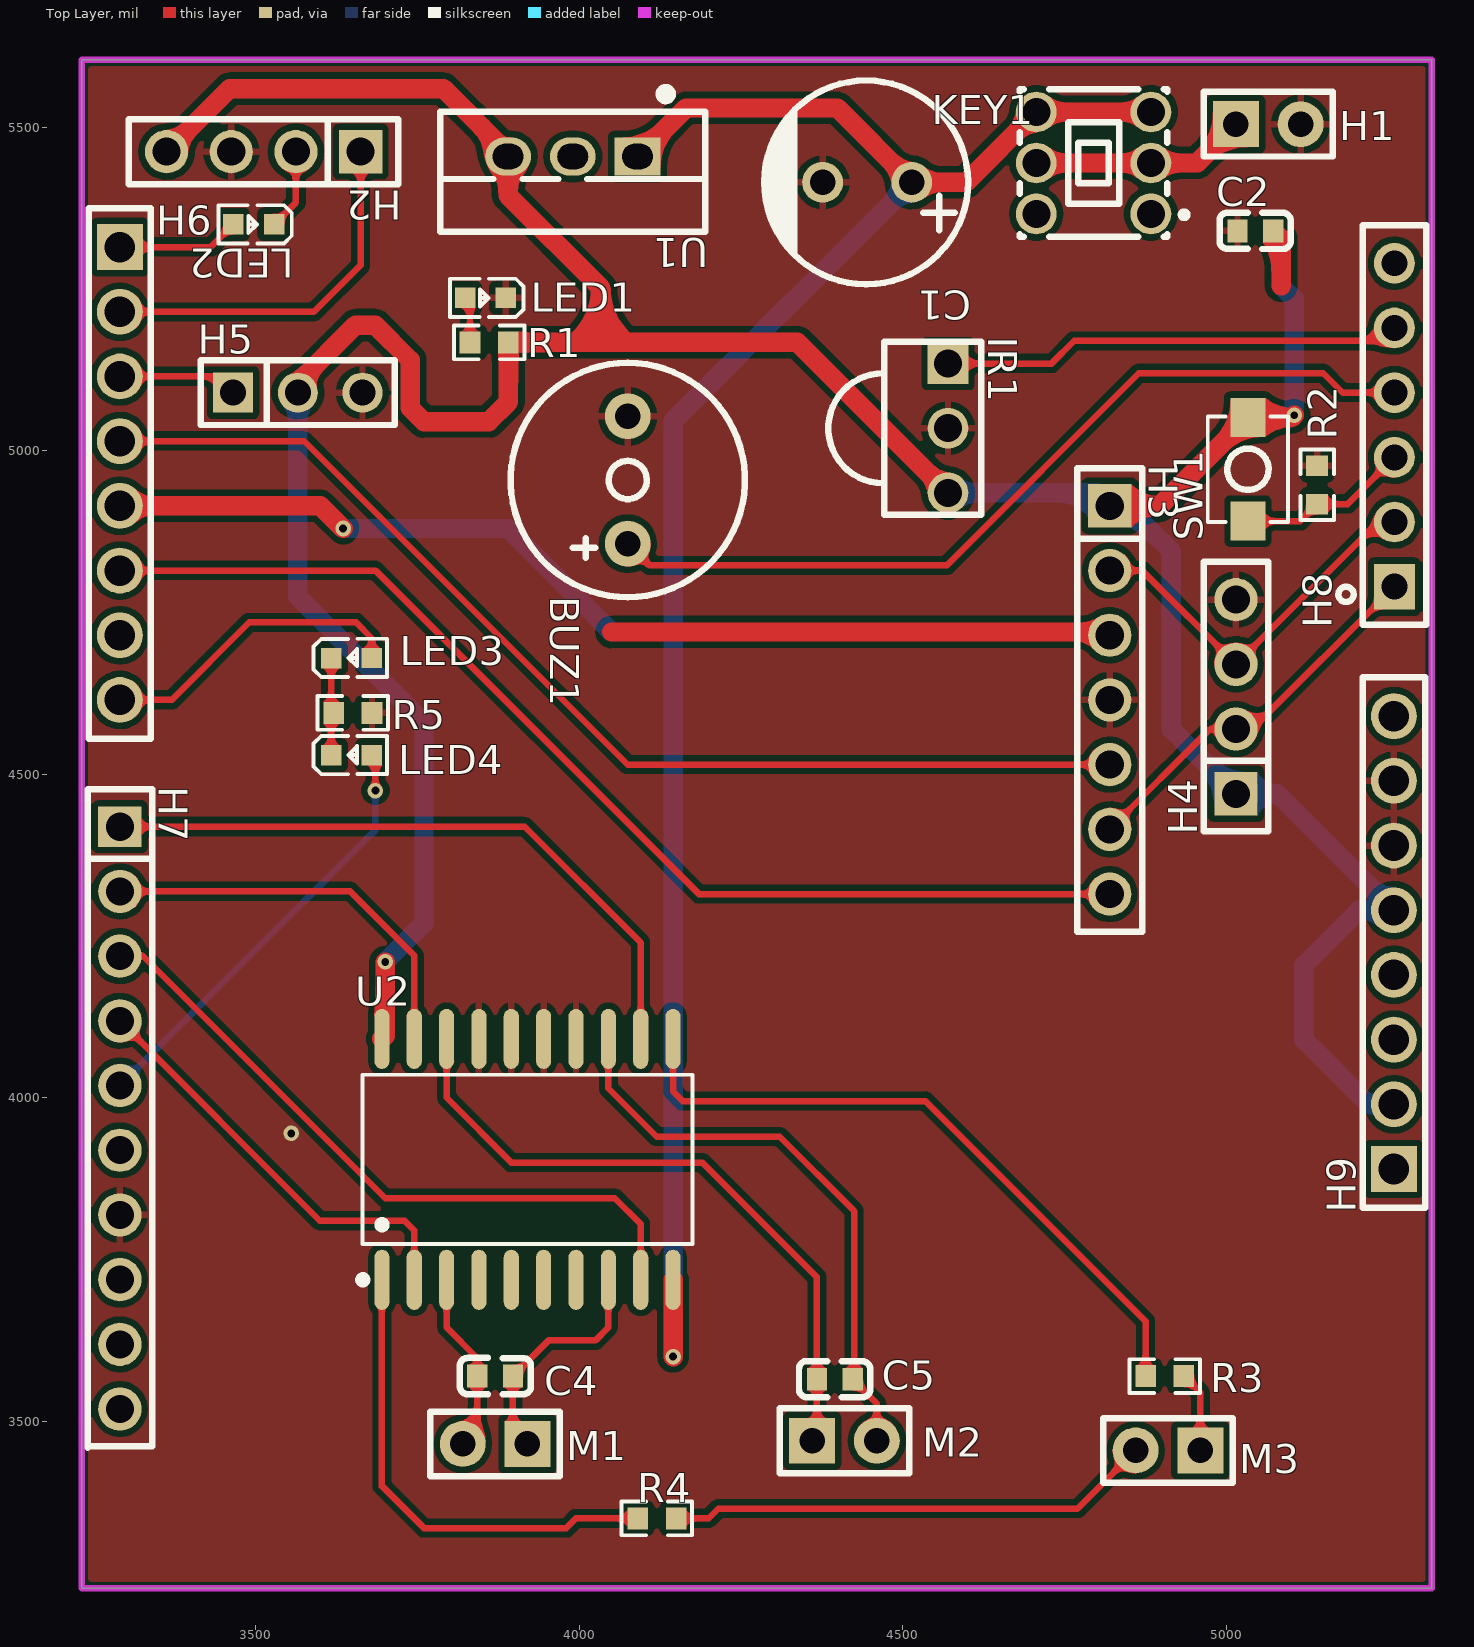
[diagram p0: Top Layer view]
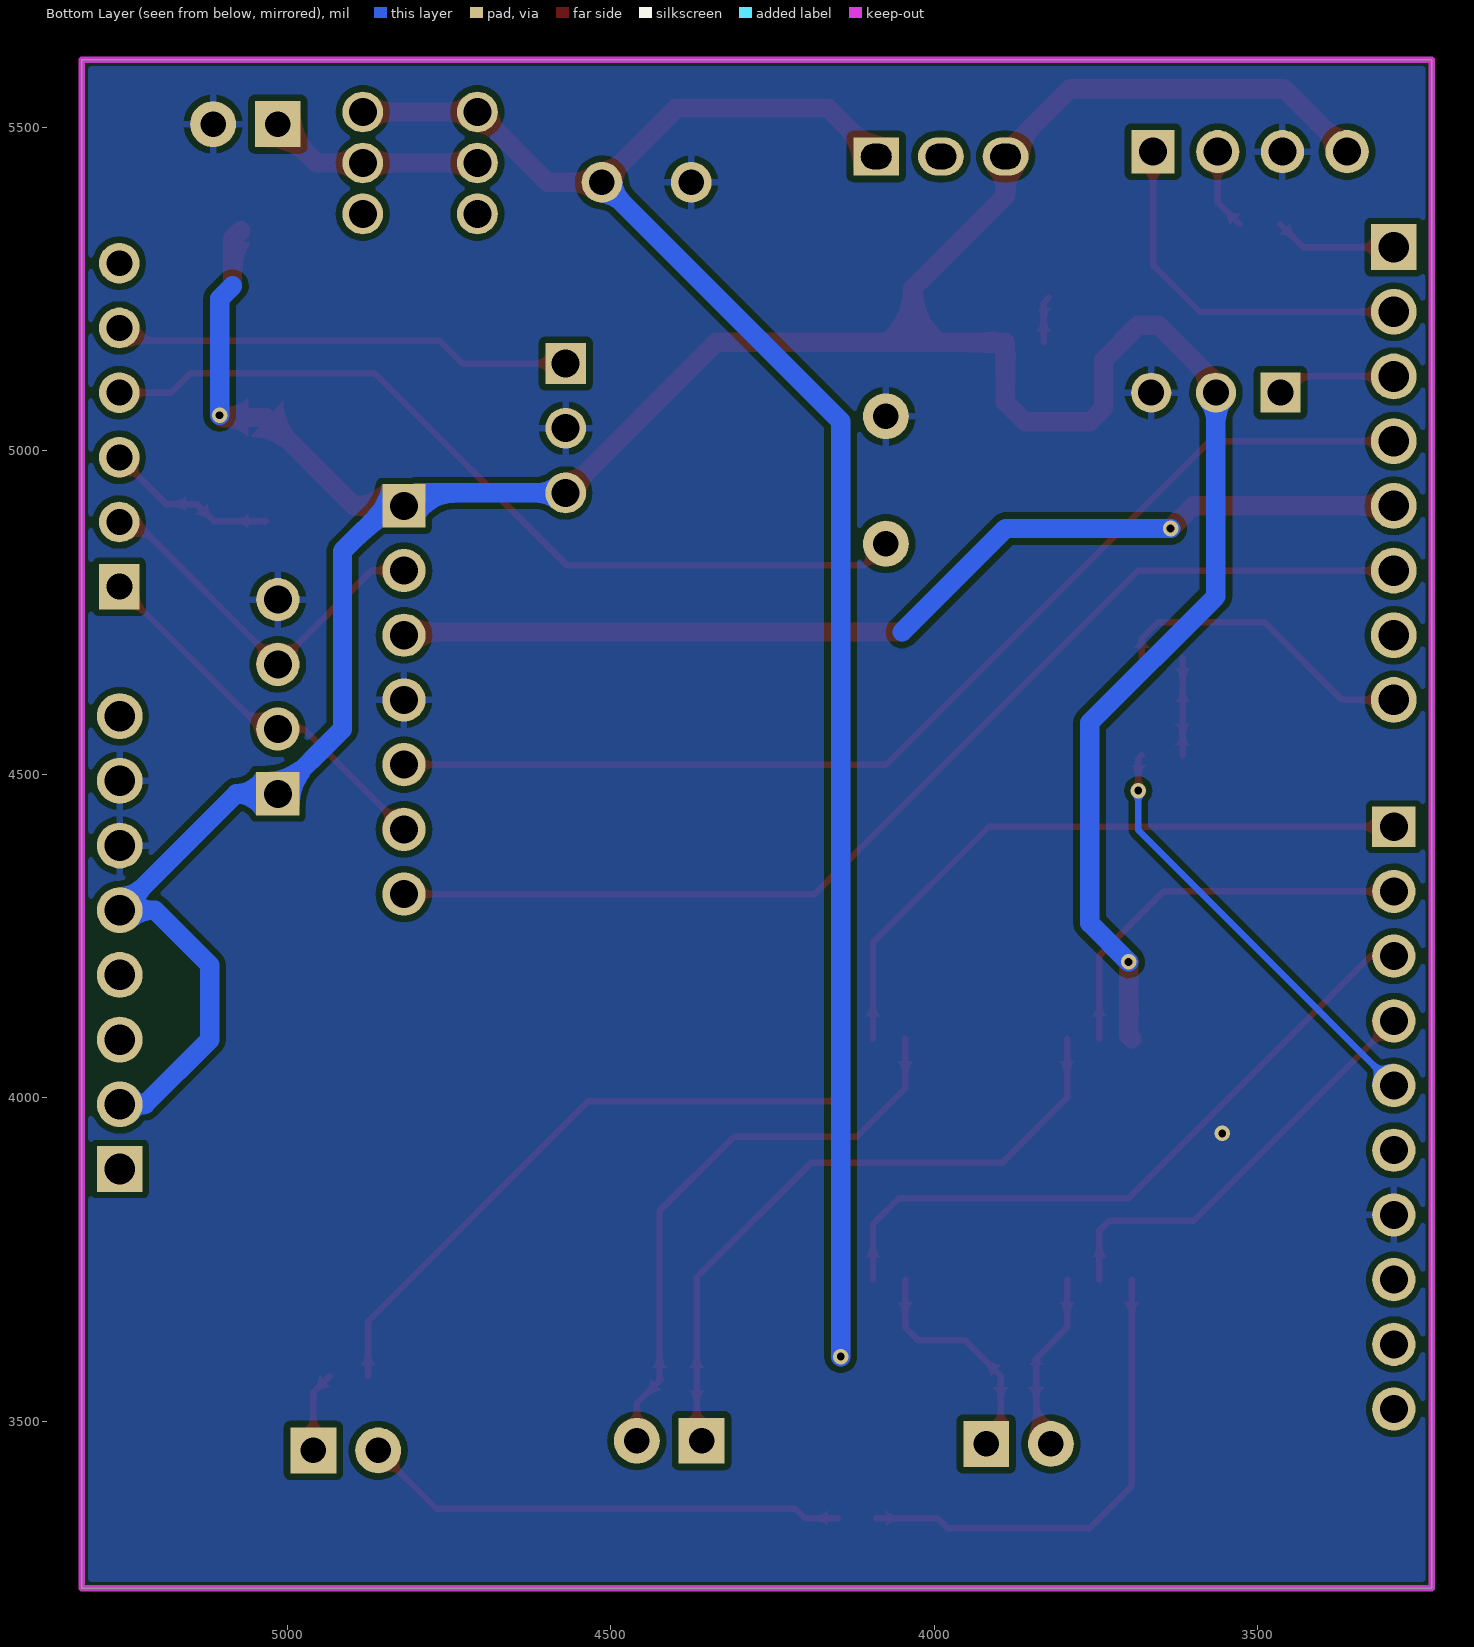
[diagram p1: Bottom Layer view, seen from below]
# Altium PCB MISC51932.pcbdoc
Units mil, origin at the board's own origin, x right, y up, seen from the top; angles counter-clockwise.
Board outline 2086.61 x 2362.2 mil, 2 copper layers (Top Layer, Bottom Layer), stack 62.206 mil thick; 31 components, 32 nets, 120 pads, 6 vias.

## Layer stack, top to bottom
Top Solder Mask Layer: solder mask 0.394, Dk 3.3
Top Layer: signal copper 1.379
Dielectric1: surface 59.449, FR4, Dk 4.5
Bottom Layer: signal copper 1.378
Bottom Solder Mask Layer: solder mask 0.394, Dk 3.3

## Board outline
5317.83,5604.37 3231.22,5604.37 3231.22,3242.17 5317.83,3242.17

## Design rules (kind name [scope] priority, off if disabled: settings)
BoardOutlineClearance copperThickness2oz_1 [All] p2 off: genericclearance=7.99 ignorepadtopadclearanceinfootprint=FALSE except(0: Arc-SplitContinuation Track-SplitContinuation SMDPad-SplitContinuation THPad-SplitContinuation Via-SplitContinuation Fill-SplitContinuation Region-SplitContinuation Poly-SplitContinuation Text-SplitContinuation Hole-SplitContinuation; 5.98: Arc-CutoutEdge Track-CutoutEdge SMDPad-CutoutEdge THPad-CutoutEdge Via-CutoutEdge Text-CutoutEdge; 6.9: Hole-OutlineEdge Hole-CutoutEdge; 10: Poly-OutlineEdge Poly-CutoutEdge; 11.81: Arc-OutlineEdge Track-OutlineEdge SMDPad-OutlineEdge THPad-OutlineEdge Via-OutlineEdge Fill-OutlineEdge Region-OutlineEdge Text-OutlineEdge Fill-CutoutEdge Region-CutoutEdge)
BoardOutlineClearance Plane_innerPlane_1 [All] p4 off: genericclearance=4.02 ignorepadtopadclearanceinfootprint=FALSE except(0: Arc-SplitContinuation Track-SplitContinuation SMDPad-SplitContinuation THPad-SplitContinuation Via-SplitContinuation Fill-SplitContinuation Region-SplitContinuation Poly-SplitContinuation Text-SplitContinuation Hole-SplitContinuation; 5.98: Arc-CutoutEdge Track-CutoutEdge SMDPad-CutoutEdge THPad-CutoutEdge Via-CutoutEdge Text-CutoutEdge; 6.9: Hole-OutlineEdge Hole-CutoutEdge; 10: Poly-OutlineEdge Poly-CutoutEdge; 11.81: Arc-OutlineEdge Track-OutlineEdge SMDPad-OutlineEdge THPad-OutlineEdge Via-OutlineEdge Fill-OutlineEdge Region-OutlineEdge Text-OutlineEdge Fill-CutoutEdge Region-CutoutEdge)
BoardOutlineClearance Copper_copperRegion_1 [All] p6 off: genericclearance=4.02 ignorepadtopadclearanceinfootprint=FALSE except(0: Arc-SplitContinuation Track-SplitContinuation SMDPad-SplitContinuation THPad-SplitContinuation Via-SplitContinuation Fill-SplitContinuation Region-SplitContinuation Poly-SplitContinuation Text-SplitContinuation Hole-SplitContinuation; 5.98: Arc-CutoutEdge Track-CutoutEdge SMDPad-CutoutEdge THPad-CutoutEdge Via-CutoutEdge Text-CutoutEdge; 6.9: Hole-OutlineEdge Hole-CutoutEdge; 10: Poly-OutlineEdge Poly-CutoutEdge; 11.81: Arc-OutlineEdge Track-OutlineEdge SMDPad-OutlineEdge THPad-OutlineEdge Via-OutlineEdge Fill-OutlineEdge Region-OutlineEdge Text-OutlineEdge Fill-CutoutEdge Region-CutoutEdge)
BoardOutlineClearance copperThickness1oz_1 [All] p8: genericclearance=4.02 ignorepadtopadclearanceinfootprint=FALSE except(0: Arc-SplitContinuation Track-SplitContinuation SMDPad-SplitContinuation THPad-SplitContinuation Via-SplitContinuation Fill-SplitContinuation Region-SplitContinuation Poly-SplitContinuation Text-SplitContinuation Hole-SplitContinuation; 5.98: Arc-CutoutEdge Track-CutoutEdge SMDPad-CutoutEdge THPad-CutoutEdge Via-CutoutEdge Text-CutoutEdge; 6.9: Hole-OutlineEdge Hole-CutoutEdge; 10: Poly-OutlineEdge Poly-CutoutEdge; 11.81: Arc-OutlineEdge Track-OutlineEdge SMDPad-OutlineEdge THPad-OutlineEdge Via-OutlineEdge Fill-OutlineEdge Region-OutlineEdge Text-OutlineEdge Fill-CutoutEdge Region-CutoutEdge)
Clearance copperThickness2oz [All] p1 off: gap=7.99 ignorepadtopadclearanceinfootprint=FALSE except(5.98: SMDPad-Track SMDPad-SMDPad THPad-Track SMDPad-THPad THPad-THPad Track-Via SMDPad-Via THPad-Via Via-Via Fill-SMDPad Region-SMDPad Fill-THPad Region-THPad Fill-Via Region-Via Fill-Fill Fill-Region Region-Region Arc-Track Arc-SMDPad Arc-THPad Arc-Via Fill-Arc Region-Arc Arc-Arc Text-Track SMDPad-Text Text-THPad Text-Via Fill-Text Region-Text Arc-Text Text-Text; 6.9: Hole-Track Hole-SMDPad Hole-THPad Hole-Via Fill-Hole Region-Hole Hole-Arc Hole-Text; 10: Poly-Track Poly-SMDPad Poly-THPad Poly-Via Poly-Fill Poly-Region Poly-Poly Poly-Arc Poly-Text Poly-Hole; 11.81: Fill-Track Region-Track)
Clearance Plane_innerPlane [All] p3 off: gap=4.02 ignorepadtopadclearanceinfootprint=FALSE except(5.98: SMDPad-Track SMDPad-SMDPad THPad-Track SMDPad-THPad THPad-THPad Track-Via SMDPad-Via THPad-Via Via-Via Fill-SMDPad Region-SMDPad Fill-THPad Region-THPad Fill-Via Region-Via Fill-Fill Fill-Region Region-Region Arc-Track Arc-SMDPad Arc-THPad Arc-Via Fill-Arc Region-Arc Arc-Arc Text-Track SMDPad-Text Text-THPad Text-Via Fill-Text Region-Text Arc-Text Text-Text; 6.9: Hole-Track Hole-SMDPad Hole-THPad Hole-Via Fill-Hole Region-Hole Hole-Arc Hole-Text; 10: Poly-Track Poly-SMDPad Poly-THPad Poly-Via Poly-Fill Poly-Region Poly-Poly Poly-Arc Poly-Text Poly-Hole; 11.81: Fill-Track Region-Track)
Clearance Copper_copperRegion [All] p5 off: gap=4.02 ignorepadtopadclearanceinfootprint=FALSE except(5.98: SMDPad-Track SMDPad-SMDPad THPad-Track SMDPad-THPad THPad-THPad Track-Via SMDPad-Via THPad-Via Via-Via Fill-SMDPad Region-SMDPad Fill-THPad Region-THPad Fill-Via Region-Via Fill-Fill Fill-Region Region-Region Arc-Track Arc-SMDPad Arc-THPad Arc-Via Fill-Arc Region-Arc Arc-Arc Text-Track SMDPad-Text Text-THPad Text-Via Fill-Text Region-Text Arc-Text Text-Text; 6.9: Hole-Track Hole-SMDPad Hole-THPad Hole-Via Fill-Hole Region-Hole Hole-Arc Hole-Text; 10: Poly-Track Poly-SMDPad Poly-THPad Poly-Via Poly-Fill Poly-Region Poly-Poly Poly-Arc Poly-Text Poly-Hole; 11.81: Fill-Track Region-Track)
Clearance copperThickness1oz [All] p7: gap=4.02 ignorepadtopadclearanceinfootprint=FALSE except(5.98: SMDPad-Track SMDPad-SMDPad THPad-Track SMDPad-THPad THPad-THPad Track-Via SMDPad-Via THPad-Via Via-Via Fill-SMDPad Region-SMDPad Fill-THPad Region-THPad Fill-Via Region-Via Fill-Fill Fill-Region Region-Region Arc-Track Arc-SMDPad Arc-THPad Arc-Via Fill-Arc Region-Arc Arc-Arc Text-Track SMDPad-Text Text-THPad Text-Via Fill-Text Region-Text Arc-Text Text-Text; 6.9: Hole-Track Hole-SMDPad Hole-THPad Hole-Via Fill-Hole Region-Hole Hole-Arc Hole-Text; 10: Poly-Track Poly-SMDPad Poly-THPad Poly-Via Poly-Fill Poly-Region Poly-Poly Poly-Arc Poly-Text Poly-Hole; 11.81: Fill-Track Region-Track)
DiffPairsRouting differentialPair [All] p1: maxlimit=6 minlimit=6 mostfreqgap=6 toplayer_minwidth=5 toplayer_prefwidth=10 toplayer_maxwidth=100 toplayer_mingap=6 toplayer_prefgap=6 toplayer_maxgap=6 bottomlayer_minwidth=5 bottomlayer_prefwidth=10 bottomlayer_maxwidth=100 bottomlayer_mingap=6 bottomlayer_prefgap=6 bottomlayer_maxgap=6 maxuncoupledlength=10
HoleToHoleClearance otherClearance [All] p1: gap=11.81 allowstackedmicrovias=TRUE
Length netLength [All] p1: minlimit=0 maxlimit=0
PasteMaskExpansion pasteMaskExpansion [All] p1: expansion=0
PlaneConnect innerPlane [All] p1: planeconnectstyle=Relief reliefexpansion=20 reliefentries=4 reliefconductorwidth=10 reliefairgap=10
PolygonConnect copperRegion [All] p1: connectstyle=Relief reliefconductorwidth=10 reliefentries=4 polygonreliefangle="90 Angle" airgapwidth=10 via.connectstyle=Relief via.reliefconductorwidth=10 via.reliefentries=4 via.polygonreliefangle="90 Angle" via.airgapwidth=10
RoutingVias viaSize [All] p1: holewidth=12.01 width=24.02 viastyle="Through Hole" minholewidth=11.81 minwidth=19.68 maxholewidth=248.03 maxwidth=393.7
SolderMaskExpansion solderMaskExpansion [IsVia] p1: expansion=-1000 istentingtop=TRUE
SolderMaskExpansion solderMaskExpansion [All] p2: expansion=2 istentingtop=FALSE
Width copperThickness2oz_2 [All] p1 off: maxlimit=100 minlimit=8 preferedwidth=10
Width copperThickness1oz_2 [All] p2: maxlimit=100 minlimit=5 preferedwidth=10

## Components (designator, comment, footprint, x,y, rotation, side; value= is the part's Value field where it differs from the comment)
BUZ1 "蜂鸣器" BUZ-TH_BD9.0-P5.00-D0.6-FD 4075,4955 r90 top
C1 "1000uF" CAP-TH_BD8.0-P3.50-D0.6-FD 4445,5415 r180 top
C2 "100nF" C0603 5045,5340 r0 top
C4 "100nF" C0603 3870,3570 r180 top
C5 "100nF" C0603 4395,3565 r0 top
H1 "" HDR-TH_2P-P2.54-V-M-1 5065,5505 r0 top
H2 "" HDR-TH_4P-P2.54-V-F 3512.13,5462.4 r180 top
H3 "" HDR-TH_7P-P2.54-V-M 4820,4615 r270 top
H4 "" HDR-TH_4P-P2.54-V-F 5015,4620 r90 top
H5 "" HDR-TH_3P-P2.54-V-F 3565,5090 r0 top
H6 "" HDR-TH_8P-P2.54-V-F-1 3290,4965 r270 top
H7 "" HDR-TH_10P-P2.54-V-F 3290,3969.02 r270 top
H8 "" HDR-TH_6P-P2.54-V-F 5260,5040 r90 top
H9 "" HDR-TH_8P-P2.54-V-F-1 5259.27,4240 r90 top
IR1 "IRM-8601M2(GPS)" SENSOR-TH_IRM-8601 4570,5035 r270 top
KEY1 "自锁开关 5.8Z白灰白260G" SW-TH_6P-L5.8-W5.8-P2.00-LS4.5-TR 4795,5445 r270 top
LED1 "" LED_0603 3853.12,5236.36 r180 top
LED2 "" LED_0603 3495,5350 r180 top
LED3 "" LED_0603 3650,4680 r0 top
LED4 "" LED_0603 3650,4530 r0 top
M1 "" HDR-TH_2P-P2.54-V-M-1 3870,3465 r180 top
M2 "" HDR-TH_2P-P2.54-V-M-1 4410,3470 r0 top
M3 "" HDR-TH_2P-P2.54-V-M-1 4910,3455 r180 top
R1 "4.7K" R0603 3860.83,5167.59 r0 top
R2 "4.7K" R0603 5140.59,4947.46 r270 top
R3 "1K" R0603 4905,3570 r0 top
R4 "1K" R0603 4120,3350 r0 top
R5 "4.7K" R0603 3650,4595 r0 top
SW1 "" Key_SMD_3x4x2 5033.58,4971.53 r90 top
U1 "7805" TO-220-3_L10.2-W4.5-P2.54-L-1 3990,5455 r180 top
U2 "L293DD" SOIC-20_L13.0-W7.6-P1.27-LS10.3-BL 3920,3905 r0 top

## Footprints (in the part's own frame and the unit in brackets; to place one, negate y for a bottom-side part, rotate by r counter-clockwise, add the part's x,y. Pads: shape width x height; smd on the part's side, far side on the other; paste and mask are expansions set on the pad)
BUZ-TH_BD9.0-P5.00-D0.6-FD [mm]
  round 1.8 hole 1 copper offset 0,0: 1(-2.5,0)
  round 1.8 hole 1: 2(2.5,0)
  silkscreen extent -4.6,-4.6 4.6,4.6
C0603 [mm]
  rect 0.8x0.9 smd: 1(-0.7,0) 2(0.7,0)
  silkscreen extent -1.41,-0.71 1.39,0.72
CAP-TH_BD8.0-P3.50-D0.6-FD [mm]
  round 1.6 hole 1: 1(-1.75,0) 2(1.75,0)
  silkscreen extent -3.96,-4 4.04,4
HDR-TH_2P-P2.54-V-M-1 [mm]
  rect 1.8x1.8 hole 1: 1(-1.27,0)
  round 1.8 hole 1: 2(1.27,0)
  silkscreen extent -2.54,-1.27 2.54,1.27
HDR-TH_3P-P2.54-V-F [mil]
  rect 62x62 hole 40.16: 1(-100,0)
  round 62 hole 40.16: 2(0,0) 3(100,0)
  silkscreen extent -150,-50 150,50
HDR-TH_4P-P2.54-V-F [mm]
  rect 1.7x1.7 hole 1.1: 1(-3.81,0)
  round 1.7 hole 1.1: 2(-1.27,0) 3(1.27,0) 4(3.81,0)
  silkscreen extent -5.29,-1.27 5.29,1.27
HDR-TH_6P-P2.54-V-F [mm]
  rect 1.8x1.6 hole 1.02: 1(-6.35,0)
  round 1.6 hole 1.02: 2(-3.81,0) 3(-1.27,0) 4(1.27,0) 5(3.81,0) 6(6.35,0)
  silkscreen extent -7.85,-1.25 7.85,2.2
HDR-TH_7P-P2.54-V-M [mm]
  rect 1.7x1.7 hole 1.1: 1(-7.62,0)
  round 1.7 hole 1.1: 2(-5.08,0) 3(-2.54,0) 4(0,0) 5(2.54,0) 6(5.08,0) 7(7.62,0)
  silkscreen extent -9.1,-1.27 9.1,1.27
HDR-TH_8P-P2.54-V-F-1 [mm]
  rect 1.8x1.8 hole 1.2: 1(-8.89,0)
  round 1.8 hole 1.2: 2(-6.35,0) 3(-3.81,0) 4(-1.27,0) 5(1.27,0) 6(3.81,0) 7(6.35,0) 8(8.89,0)
  silkscreen extent -10.41,-1.22 10.41,1.22
HDR-TH_10P-P2.54-V-F [mm]
  rect 1.575x1.7 hole 1.1: 1(-11.43,0)
  round 1.7 hole 1.1: 2(-8.89,0) 3(-6.35,0) 4(-3.81,0) 5(-1.27,0) 6(1.27,0) 7(3.81,0) 8(6.35,0) 9(8.89,0) 10(11.43,0)
  silkscreen extent -12.9,-1.27 12.95,1.27
Key_SMD_3x4x2 [mm]
  rect 1.53x1.36 smd paste+0 mask+0.051: 1(-2.035,0) 2(2.035,0)
  silkscreen extent -2.08,-1.58 2.08,1.58
LED_0603 [mil]
  rect 31.5x31.5 smd paste+0 mask+2: 1(-33.5,-0.4) 2(29.5,-0.2)
  silkscreen extent -61,-30 53,30
R0603 [mil]
  rect 31.75x34.02 smd paste-3937.01 mask+2: 1(-29.66,0) 2(29.66,0)
  silkscreen extent -55,-26 55,26
SENSOR-TH_IRM-8601 [mm]
  rect 1.6x1.6 hole 1.1: 1(-2.54,0)
  round 1.6 hole 1.1: 2(0,0) 3(2.54,0)
  silkscreen extent -3.4,-4.7 3.4,1.3
SOIC-20_L13.0-W7.6-P1.27-LS10.3-BL [mm]
  oval 0.595x2.36 smd: 1(-5.715,-4.73) 2(-4.445,-4.73) 3(-3.175,-4.73) 4(-1.905,-4.73) 5(-0.635,-4.73) 6(0.635,-4.73) 7(1.905,-4.73) 8(3.175,-4.73) 9(4.445,-4.73) 10(5.715,-4.73) 11(5.715,4.73) 12(4.445,4.73) 13(3.175,4.73) 14(1.905,4.73) 15(0.635,4.73) 16(-0.635,4.73) 17(-1.905,4.73) 18(-3.175,4.73) 19(-4.445,4.73) 20(-5.715,4.73)
  silkscreen extent -6.61,-4.88 6.48,3.32
SW-TH_6P-L5.8-W5.8-P2.00-LS4.5-TR [mm]
  round 1.6 hole 1.1: 1(2,2.25) 2(0,2.25) 3(-2,2.25) 4(-2,-2.25) 5(0,-2.25) 6(2,-2.25)
  silkscreen extent -2.9,-2.9 2.9,3.68
TO-220-3_L10.2-W4.5-P2.54-L-1 [mm]
  rect 1.8x1.5 hole 1 slot 1.2 at 0 deg: 1(-2.54,0)
  oval 1.8x1.5 hole 1 slot 1.2 at 0 deg: 2(0,0) 3(2.54,0)
  silkscreen extent -5.2,-2.65 5.2,2.95

## Via types
v1: diameter 24, hole 12, Top Layer to Bottom Layer, 5 vias
v2: diameter 24.02, hole 12, Top Layer to Bottom Layer, 1 vias

## Nets (pads, with @x,y where several pads share a name; then routed paths per layer and width w, separated by ;. In a path a pad name is that pad's centre, name@x,y a point inside that pad or via, vN(x,y) a via of type N, cw(c..) or ccw(c..) an arc to the next point about the centre after c; other vN are vias at no path point)
$1N326: LED1.2 R1.1 | length 72.1
  Top Layer w10: LED1.2 3831.17,5229.01 R1.1
$1N838: H1.1 KEY1.2 KEY1.5 | length 333.4
  Top Layer w30: KEY1.5 KEY1.2 4955,5445 H1.1
$1N1064: H2.2 LED2.1 | length 125.9
  Top Layer w10: LED2.1 3562.13,5384.03 H2.2
$1N2239: C4.1 M1.1 U2.8 | length 366.6
  Top Layer w10: M1.1 3897.56,3487.44 C4.1 3952.56,3625 4025,3625 4045,3645 U2.8
$1N2244: C4.2 M1.2 U2.3 | length 282.7
  Top Layer w10: U2.3 3795,3645 3842.44,3597.56 C4.2 3842.44,3487.44 M1.2
$1N2373: C5.1 M2.1 U2.18 | length 1034.2
  Top Layer w10: U2.18 3795,4000 3895,3900 4190,3900 4367.44,3722.56 C5.1 4367.44,3477.44 M2.1
$1N2377: C5.2 M2.2 U2.13 | length 906.4
  Top Layer w10: U2.13 4045,4015 4120,3940 4310,3940 4425,3825 4425,3567.44 C5.2 4460,3527.56 M2.2
$1N2532: R4.1 U2.1 | length 747.3
  Top Layer w10: U2.1 3695,3400 3760,3335 3980,3335 3995,3350 R4.1
$1N2537: R3.1 U2.11 | length 1043.4
  Top Layer w10: U2.11 4145,4010 4160,3995 4535,3995 4875.34,3654.66 R3.1
$1N2566: M3.1 R3.2 | length 125.5
  Top Layer w10: R3.2 4960,3544.66 M3.1
$1N2602: M3.2 R4.2 | length 753.8
  Top Layer w10: R4.2 4200,3350 4215,3365 4770,3365 M3.2
$1N3024: H6.8 LED3.2 | length 480.1
  Top Layer w10: H6.8 3370,4615 3490,4735 3655,4735 3679.5,4710.5 LED3.2
$1N3068: H7.5 LED4.2 | length 676.7
  Top Layer w10: LED4.2 3685,4524.3 v1(3685,4475)
  Bottom Layer w10: H7.5 3685,4414.02 v1(3685,4475)
$1N3103: LED3.1 LED4.1 R5.1 | length 150
  Top Layer w10: LED4.1 LED3.1
A0: H3.6 H4.2 H8.1 | length 595.3
  Top Layer w10: H3.6 4975,4570 H4.2 5040,4570 H8.1
A1: H3.2 H4.3 H8.2 | length 591.2
  Top Layer w10: H3.2 4870,4815 H4.3 5235,4890 H8.2
A4: H8.5 IR1.1 | length 712.8
  Top Layer w10: IR1.1 4730,5135 4765,5170 5240,5170 H8.5
BEEP: BUZ1.1 H8.4 | length 1334.4
  Top Layer w10: BUZ1.1 4108.65,4822.93 4567.93,4822.93 4865,5120 5150,5120 5180,5090 H8.4
D2: H5.1 H6.3 | length 185.4
  Top Layer w10: H6.3 3440,5115 H5.1
D3: H3.5 H6.4 | length 1737.1
  Top Layer w10: H6.4 3575,5015 4075,4515 H3.5
D4: H3.3 H6.5 | length 1612.8
  Top Layer w30: H6.5 3600,4915 v1(3635,4880) ; 4050,4720 4815,4720 H3.3
  Bottom Layer w30: v1(3635,4880) 3890,4880 4050,4720
D5: H3.7 H6.6 | length 1737.1
  Top Layer w10: H6.6 3685,4815 4185,4315 H3.7
GND: BUZ1.2 C1.2 C2.1 H1.2 H2.3 H3.4 H4.4 H5.3 H7.7 H9.6 H9.7 IR1.2 LED1.1 R2.1 R5.2 U2.14 U2.15 U2.16 U2.17
  other v2: 3555,3945
INBAT: C1.1 KEY1.3 KEY1.4 U1.1 U2.10 | length 3003.9
  Top Layer w30: U1.1 4165,5530 4398.9,5530 C1.1 4597.68,5415 KEY1.4 KEY1.3 ; v1(4145,3600) U2.10
  Bottom Layer w30: v1(4145,3600) 4145,5046.1 C1.1
INPUT1: H7.4 U2.2 | length 665.4
  Top Layer w10: H7.4 3599.02,3810 3730,3810 3745,3795 U2.2
INPUT2: H7.3 U2.9 | length 1062.7
  Top Layer w10: H7.3 3325.98,4219.02 3700,3845 4055,3845 4095,3805 U2.9
INPUT3: H7.1 U2.12 | length 1027.9
  Top Layer w10: H7.1 3915.98,4419.02 4095,4240 U2.12
INPUT4: H7.2 U2.19 | length 624.8
  Top Layer w10: H7.2 3645.98,4319.02 3745,4220 U2.19
KEY: H8.3 R2.2 SW1.1 | length 267.3
  Top Layer w10: SW1.1 5114.19,4891.41 R2.2 5187.8,4917.8 H8.3
RXD: H6.1 LED2.2 | length 190.1
  Top Layer w10: H6.1 3430.3,5315 LED2.2
TXD: H2.1 H6.2 | length 577.3
  Top Layer w10: H6.2 3590,5215 3662.13,5287.13 H2.1
VCCBAT: C2.2 H2.4 H3.1 H4.1 H5.2 H9.2 H9.5 IR1.3 R1.2 SW1.2 U1.3 U2.20 | length 5660.3
  Top Layer w30: H2.4 3459.73,5560 3790,5560 3890,5460 U1.3 3890,5395 4033.39,5251.61 4033.39,5167.59 ; H5.2 3565,5105 3654.39,5194.39 3684.39,5194.39 3738.79,5140 3738.79,5066.21 3760,5045 3860,5045 3890.49,5075.49 R1.2 4033.39,5167.59 ; U2.20 3700,4096.22 v1(3700,4210) ; IR1.3 4337.41,5167.59 4033.39,5167.59 ; H3.1 4896.94,4915 SW1.2 5101.65,5051.65 v1(5105,5055) ; C2.2 5085,5327.56 5085,5255
  Bottom Layer w30: H5.2 3565,4775 3760,4580 3760,4270 v1(3700,4210) ; IR1.3 4800,4935 H3.1 4845,4915 4915,4845 4915,4570 H4.1 5079.27,4470 H9.5 5205,4290 5120,4205 5120,4090 5220,3990 H9.2 ; 5085,5255 5105,5235 v1(5105,5055)
pads on no net: H6.7 H7.6 H7.8 H7.9 H7.10 H8.6 H9.1 H9.3 H9.4 H9.8 KEY1.1 KEY1.6 U1.2 U2.4 U2.5 U2.6 U2.7

## Polygon pours and split planes (outlines as drawn)
GND on Top Layer (solid, remove dead copper, pour order 0): 3135,5700 3135,3110 5410,3110 5410,5700
GND on Bottom Layer (solid, remove dead copper, pour order 2): 3000,5785 3000,3000 5395,3000 5395,5785

## Keep-outs
Board Outline Layer:
  the board outline again, w10

## Other copper
Top Layer:
  drawing of 95 lines, arcs and shapes, not listed
Bottom Layer:
  region net $1N3068: 3690,4458.6 3680,4458.6 3679.91,4459.72 3679.66,4460.85 3678.77,4463.08 3677.5,4465.17 3676.06,4467 3693.94,4467 3692.5,4465.17 3691.23,4463.08 3690.34,4460.85 3690.09,4459.72
  region net $1N3068: 3318.8,4054.89 3325.87,4047.82 3324.11,4045.9 3322.77,4044.08 3321.79,4042.34 3321.15,4040.67 3320.78,4039.03 3320.67,4037.41 3320.75,4035.78 3320.99,4034.12 3321.77,4030.63 3322.66,4026.76 3323.32,4022.33 3323.46,4019.84 3323.41,4017.15 3288.14,4052.43 3290.83,4052.48 3293.31,4052.34 3297.74,4051.68 3301.61,4050.78 3305.11,4050.01 3306.76,4049.77 3308.39,4049.68 3310.01,4049.8 3311.65,4050.16 3313.33,4050.81 3315.06,4051.78 3316.88,4053.13
  region net VCCBAT: 4613.04,4950 4613.04,4920 4610.47,4919.81 4607.58,4919.27 4604.52,4918.44 4601.41,4917.35 4598.38,4916.07 4595.55,4914.64 4593.04,4913.11 4591,4911.52 4591,4958.48 4593.04,4956.89 4595.55,4955.36 4598.38,4953.93 4601.41,4952.65 4604.52,4951.56 4607.58,4950.73 4610.47,4950.19
  region net VCCBAT: 4741.54,4920 4741.54,4950 4764.02,4948.85 4786.54,4948.46 4786.54,4897.5 4782.33,4902.48 4777.58,4906.94 4772.34,4910.81 4766.69,4914.06 4760.7,4916.63 4754.46,4918.5 4748.04,4919.62 4741.54,4920
  region net VCCBAT: 4874.93,4906.29 4887.18,4851.61 4876.34,4862.03 4865.09,4872.01 4853.46,4881.54 4853.46,4948.46 4854.84,4941.73 4856.81,4935.15 4859.36,4928.77 4862.48,4922.65 4866.13,4916.83 4870.29,4911.36 4874.93,4906.29
  region net VCCBAT: 4965.63,4498.16 4986.84,4519.37 4992.88,4515.26 4999.28,4511.72 5005.97,4508.78 5012.91,4506.47 5020.02,4504.81 5027.27,4503.8 5034.57,4503.46 4981.54,4450.43 4981.2,4457.73 4980.19,4464.98 4978.53,4472.09 4976.22,4479.03 4973.28,4485.72 4969.74,4492.12 4965.63,4498.16
  region net VCCBAT: 5079.27,4485 5079.27,4455 5074.57,4454.68 5069.95,4453.73 5065.51,4452.17 5061.31,4450.03 5057.44,4447.34 5053.97,4444.16 5050.96,4440.53 5048.46,4436.54 5048.46,4503.46 5050.96,4499.47 5053.97,4495.84 5057.44,4492.66 5061.31,4489.97 5065.51,4487.83 5069.95,4486.27 5074.57,4485.32 5079.27,4485
  region net VCCBAT: 5214.42,4313.64 5235.63,4334.85 5238.12,4332.72 5240.99,4330.88 5244.14,4329.32 5247.5,4328.02 5250.98,4326.99 5254.49,4326.21 5257.94,4325.67 5261.24,4325.38 5223.89,4288.03 5223.6,4291.33 5223.06,4294.78 5222.28,4298.29 5221.25,4301.77 5219.95,4305.13 5218.39,4308.28 5216.55,4311.15
  region net VCCBAT: 5210.84,4275 5210.84,4305 5214.1,4305.26 5217.43,4305.98 5220.77,4307.11 5224.06,4308.57 5227.25,4310.29 5230.28,4312.22 5233.1,4314.28 5235.65,4316.41 5235.65,4263.59 5233.1,4265.72 5230.28,4267.78 5227.25,4269.71 5224.06,4271.43 5220.77,4272.89 5217.43,4274.02 5214.1,4274.74
  region net VCCBAT: 5220,3975 5220,4005 5222.87,4005.26 5225.16,4005.98 5227.03,4007.11 5228.64,4008.57 5231.71,4012.22 5233.49,4014.28 5235.65,4016.41 5235.65,3963.59 5233.49,3965.72 5231.71,3967.78 5228.64,3971.43 5227.03,3972.89 5225.16,3974.02 5222.87,3974.74
  region net INBAT: 4494.07,5373.96 4472.86,5395.17 4474.54,5397.13 4476.2,5399.55 4477.77,5402.3 4479.21,5405.27 4480.45,5408.32 4481.44,5411.33 4482.12,5414.19 4482.45,5416.75 4515.65,5383.55 4513.09,5383.22 4510.23,5382.54 4507.22,5381.55 4504.17,5380.31 4501.2,5378.87 4498.45,5377.3 4496.03,5375.64
  region net VCCBAT: 3580,5047.63 3550,5047.63 3549.82,5050.19 3549.33,5053.03 3548.55,5056.03 3547.53,5059.09 3546.31,5062.06 3544.94,5064.84 3543.45,5067.31 3541.89,5069.33 3588.11,5069.33 3586.55,5067.31 3585.06,5064.84 3583.69,5062.06 3582.47,5059.09 3581.45,5056.03 3580.67,5053.03 3580.18,5050.19